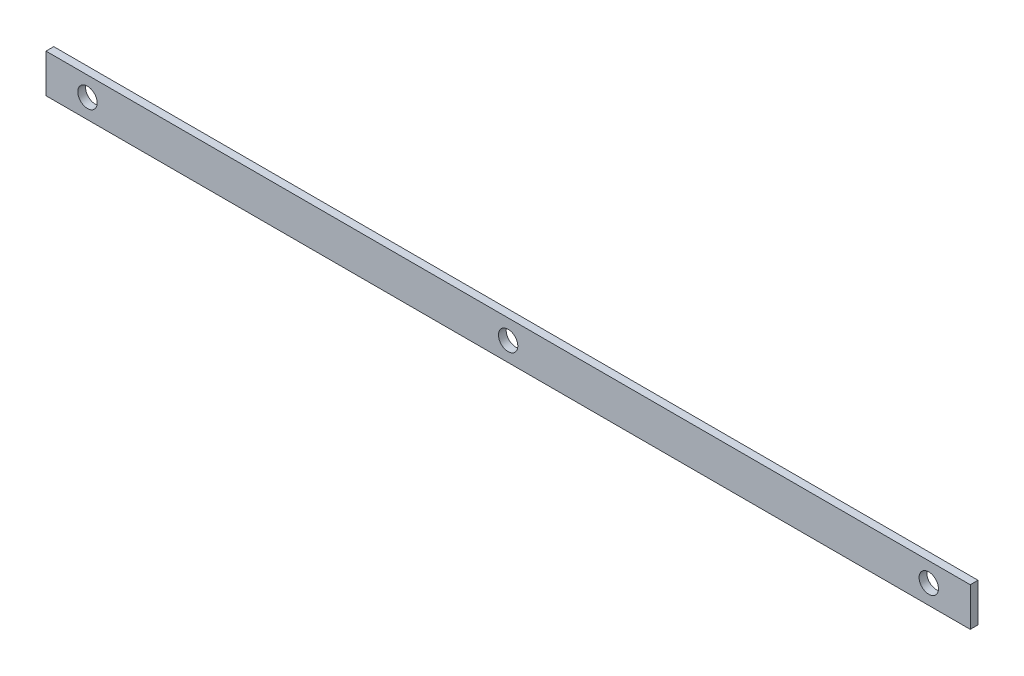
SolidWorks part; units mm, degrees
ref_plane "Front Plane" through (0, 0, 0) normal (0, 0, 1) x (1, 0, 0)
ref_plane "Top Plane" through (0, 0, 0) normal (0, 1, 0) x (1, 0, 0)
ref_plane "Right Plane" through (0, 0, 0) normal (1, 0, 0) x (0, 0, -1)
other "Configuration Table"
sketch "Sketch1" plane through (0, 0, 0) normal (0, 0, 1) x (1, 0, 0)
  line L1 (59.6548, 62.0807) -> (-59.6548, 62.0807)
  line L2 (59.6548, 62.0807) -> (59.6548, 57.0865)
  line L3 (59.6548, 57.0865) -> (-59.6548, 57.0865)
  line L4 (-59.6548, 62.0807) -> (-59.6548, 57.0865)
  line L5 (0, 57.0865) -> (0, 62.0807) construction
  line L6 (59.6548, 59.5836) -> (-59.6548, 59.5836) construction
  point P0 (0, 59.5836)
extrude "Boss-Extrude1" add sketch "Sketch1" along normal blind 1
sketch "Sketch2" plane through (0, 0, 1) normal (0, 0, 1) x (1, 0, 0)
  line L0 (-54.3003, 64.1447) -> (-54.3003, 59.5836) construction
  circle A0 centre (-54.3003, 59.5836) radius 1.25
  circle A1 centre (0, 59.5601) radius 1.25
  circle A2 centre (54.3003, 59.5836) radius 1.25
extrude "Cut-Extrude1" cut sketch "Sketch2" against normal blind 1
